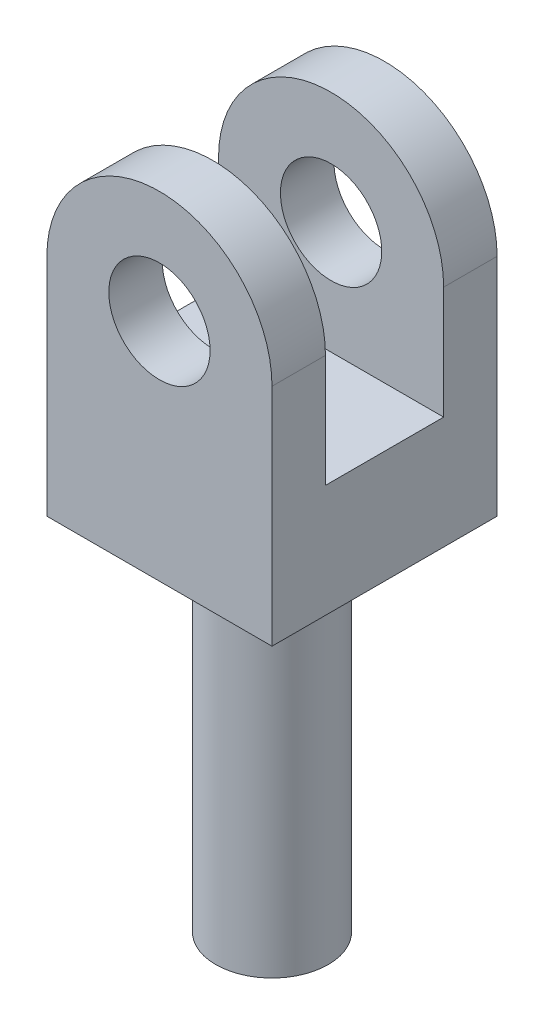
from build123d import *

# Parameters (mm, degrees)
SKETCH1_R           = 45
BOSS_EXTRUDE2_DEPTH = 200
SKETCH2_W           = 105
SKETCH2_H           = 318.049906591
CUT_EXTRUDE1_DEPTH  = 325.763563649
SKETCH3_R           = 50
BOSS_EXTRUDE3_DEPTH = 320
SKETCH4_R           = 25
CUT_EXTRUDE2_DEPTH  = 100
FILLET1_R           = 10


with BuildPart() as part:
    # Sketch1 → Boss-Extrude2 (new body)
    with BuildSketch(Plane.XY):
        with BuildLine():
            Line((140.402467833, -159.597532167), (-59.597532167, -159.597532167))
            Line((-59.597532167, -159.597532167), (-59.597532167, 40.402467833))
            ThreePointArc((-59.597532167, 40.402467833), (40.402467833, 140.402467833), (140.402467833, 40.402467833))
            Line((140.402467833, 40.402467833), (140.402467833, -159.597532167))
        make_face()
        with Locations((40.402467833, 40.402467833)):
            Circle(SKETCH1_R, mode=Mode.SUBTRACT)
    extrude(amount=BOSS_EXTRUDE2_DEPTH)

    # Sketch2 → Cut-Extrude1 (cut, through all)
    with BuildSketch(Plane(origin=(140.402467833, 0, 0), x_dir=(0, 0, -1), z_dir=(1, 0, 0))):
        with Locations((-100, 99.427421129)):
            Rectangle(SKETCH2_W, SKETCH2_H)
    extrude(amount=-CUT_EXTRUDE1_DEPTH, mode=Mode.SUBTRACT)

    # Sketch3 → Boss-Extrude3 (add)
    with BuildSketch(Plane.XZ.offset(159.597532167)):
        with Locations((40.402467833, 100)):
            Circle(SKETCH3_R)
    extrude(amount=BOSS_EXTRUDE3_DEPTH)

    # Sketch4 → Cut-Extrude2 (cut)
    with BuildSketch(Plane.XZ.offset(479.597532167)):
        with Locations((40.402467833, 100)):
            Circle(SKETCH4_R)
    extrude(amount=-CUT_EXTRUDE2_DEPTH, mode=Mode.SUBTRACT)

    # Fillet1
    fillet1_edges = [part.edges().sort_by_distance(p)[0] for p in [
        (-9.597532167, -159.597532167, 100),
    ]]
    fillet(fillet1_edges, radius=FILLET1_R)


solid = part.part
